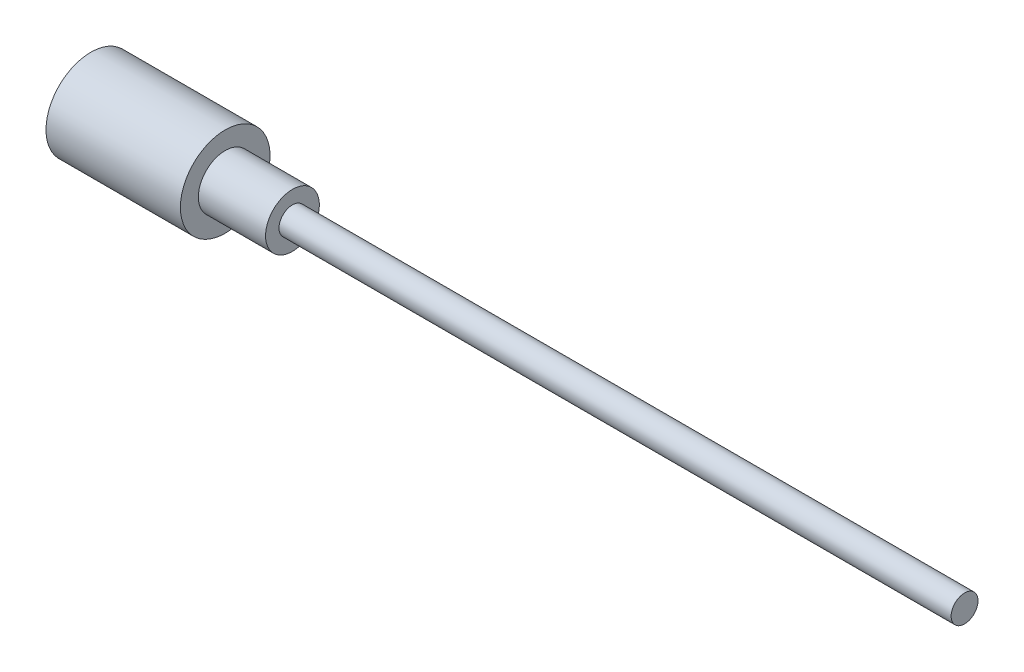
from build123d import *


with BuildPart() as part:
    # Sketch1 → Revolve1 (revolve)
    with BuildSketch(Plane.XY, mode=Mode.PRIVATE) as revolve1_sk:
        Polygon((0, 0), (0, 10), (30, 10), (30, 6), (45, 6), (45, 3), (195, 3), (195, 0), align=None)
    revolve(revolve1_sk.sketch.rotate(Axis((0, 0, 0), (1, 0, 0)), 90), axis=Axis((0, 0, 0), (1, 0, 0)))


solid = part.part
